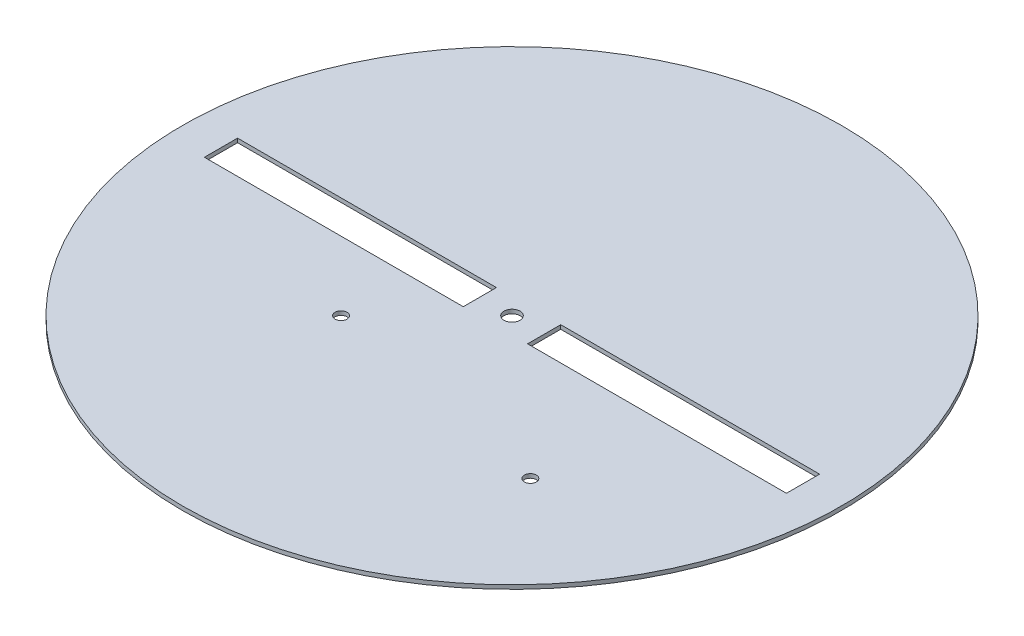
from build123d import *

# Parameters (mm, degrees)
SKETCH1_R           = 82.5
SKETCH1_R_2         = 1.5
SKETCH1_R_3         = 2
SKETCH1_W           = 64.8
SKETCH1_H           = 8.3
BOSS_EXTRUDE1_DEPTH = 1


with BuildPart() as part:
    # Sketch1 → Boss-Extrude1 (new body)
    with BuildSketch(Plane(origin=(0, 0, 0), x_dir=(1, 0, 0), z_dir=(0, 1, 0))):
        with Locations(Location((0, 0, 0), (0, 0, 270))):
            Circle(SKETCH1_R)
        with Locations(Location((-21.4, -21.4, 0), (0, 0, 270))):
            Circle(SKETCH1_R_2, mode=Mode.SUBTRACT)
        with Locations(Location((37.6, -33, 0), (0, 0, 270))):
            Circle(SKETCH1_R_2, mode=Mode.SUBTRACT)
        with Locations(Location((0, 0, 0), (0, 0, 270))):
            Circle(SKETCH1_R_3, mode=Mode.SUBTRACT)
        with Locations((-40.45, 0)):
            Rectangle(SKETCH1_W, SKETCH1_H, mode=Mode.SUBTRACT)
        with Locations((40.45, 0)):
            Rectangle(SKETCH1_W, SKETCH1_H, mode=Mode.SUBTRACT)
    extrude(amount=BOSS_EXTRUDE1_DEPTH)


solid = part.part
